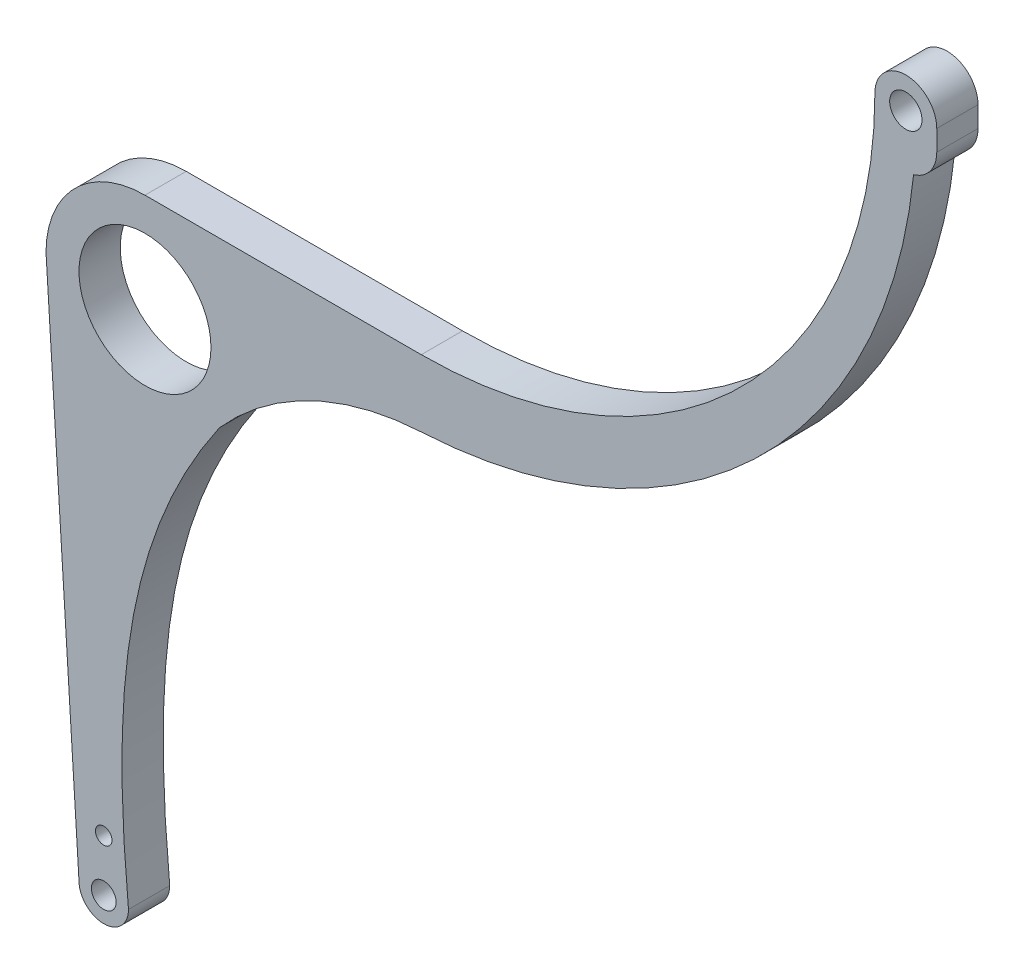
SolidWorks part; units mm, degrees
ref_plane "前视基准面" through (0, 0, 0) normal (0, 0, 1) x (1, 0, 0)
ref_plane "上视基准面" through (0, 0, 0) normal (0, 1, 0) x (1, 0, 0)
ref_plane "右视基准面" through (0, 0, 0) normal (1, 0, 0) x (0, 0, -1)
other "Configuration Table"
sketch "草图1" plane through (0, 0, 0) normal (0, 0, 1) x (1, 0, 0)
  line L0 (-60.8711, 0) -> (72.3657, 0) construction
  line L1 (-84.052, 128) -> (106.5467, 128) construction
  line L2 (0, 12.5) -> (0, -18.0859) construction
  line L3 (0, -18.0859) -> (10, -18.0859) construction
  line L4 (10, -18.0859) -> (10, 407.7959) construction
  line L5 (-9, 59.8208) -> (-9, -18.0859) construction
  line L6 (-14, 128) -> (-6, 0)
  line L7 (-176.4012, 262) -> (270.3663, 262) construction
  line L8 (77, 485.9134) -> (77, 110.3328) construction
  line L9 (10, 152) -> (77, 152)
  line L10 (187, 262) -> (194.5, 262) construction
  line L11 (202, 262) -> (202, 257)
  line L12 (202, 257) -> (194.1788, 257) construction
  line L13 (70.6056, 267.7759) -> (70.6056, 254.1409) construction
  line L14 (4.2515, 65.8248) -> (157.9856, 65.8248) construction
  line L15 (80.543, 130.5208) -> (80.543, 47.5555) construction
  line L16 (4.7446, 112.1309) -> (49.2871, 112.1309) construction
  line L17 (-29.78, 372) -> (265.8488, 372) construction
  circle A0 centre (0, 0) radius 3
  arc A1 (-6, 0) -> (6, 0) centre (0, 0) ccw
  circle A2 centre (10, 128) radius 16
  arc A3 (10, 152) -> (-14, 128) centre (10, 128) ccw
  circle A4 centre (77, 262) radius 115 construction
  arc A5 (77, 152) -> (187, 262) centre (77, 262) ccw
  arc A6 (202, 262) -> (187, 262) centre (194.5, 262) ccw
  arc A9 (196.3799, 249.4949) -> (202, 257) centre (194.1788, 257) ccw
  arc A10 (77, 135.7674) -> (28.0048, 112.1309) centre (80.543, 65.8248) ccw
  arc A11 (77, 135.7674) -> (196.3799, 249.4949) centre (70.6056, 262) ccw
  circle A12 centre (194.5, 262) radius 3.919
  circle A13 centre (0, 12.5) radius 2
  spline S0 degree 3 poles (6, 0) (1.5887, 45.6809) (5.6041, 79.6432) (28.0048, 112.1309) knots 0 0 0 0 0.788155 0.788155 0.788155 0.788155
  dimension "D1" = 6
  dimension "D2" = 12
  dimension "D5" = 19
  dimension "D6" = 134
  dimension "D8" = 230
  dimension "D9" = 6.3944
  dimension "D10" = 62.1752
  dimension "D12" = 15.8691
  dimension "D14" = 24
  dimension "D15" = 4
  dimension "D16" = 7.838
  dimension "D17" = 7.5
  dimension "D18" = 220
  dimension "D3" = 128
  dimension "D4" = 9
  dimension "D7" = 67
  dimension "D11" = 70.543
  dimension "D13" = 12.5
extrude "凸台-拉伸1" add sketch "草图1" along normal blind 10
